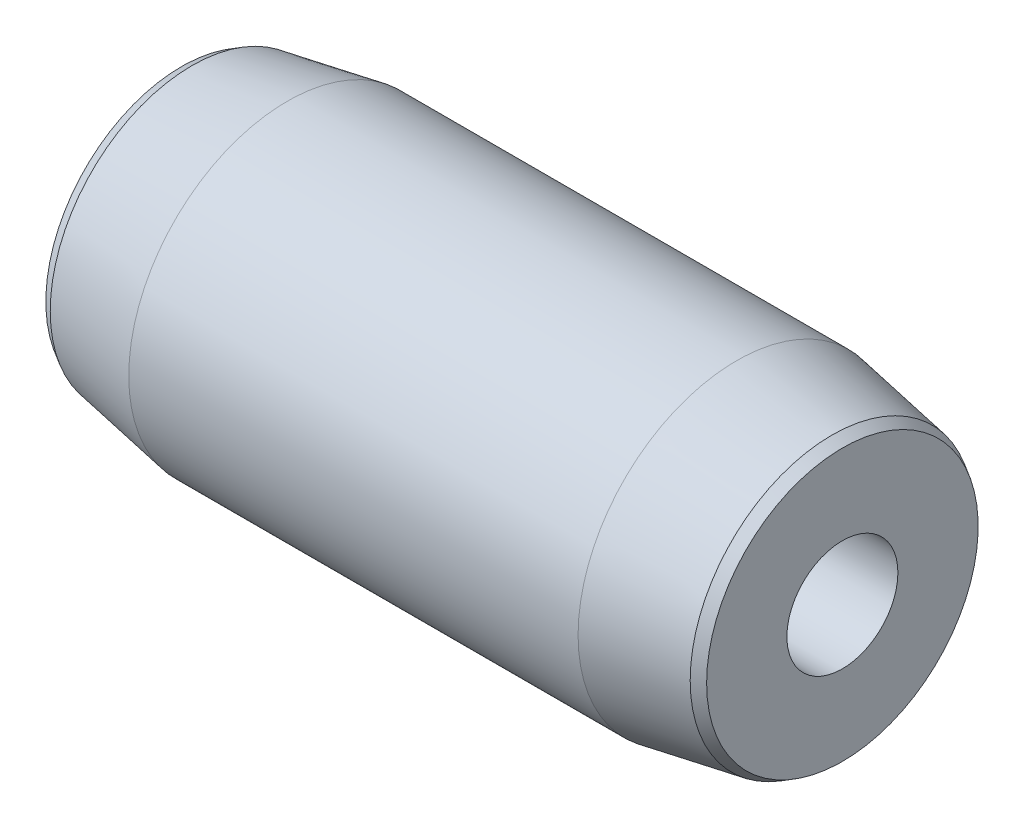
from build123d import *
from OCP.BRepFilletAPI import BRepFilletAPI_MakeChamfer

# Parameters (mm, degrees)
SKETCH_2_R              = 10.5
CUT_EXTRUDE_1_DEPTH     = 133.003787824
HOLE_WIZARD_M24_2_D     = 21
HOLE_WIZARD_M24_2_DEPTH = 63
HOLE_WIZARD_M24_2_TIP   = 6.3090365
CHAMFER_1_SIZE          = 2
CHAMFER_1_SIZE2         = 0.789861687


with BuildPart() as part:
    # 草图1 → 旋转1 (revolve)
    with BuildSketch(Plane.XY, mode=Mode.PRIVATE) as revolve_1_sk:
        Polygon((0, 0), (0, 26.473460386), (20, 30), (105, 30), (125, 26.473460386), (125, 0), align=None)
    revolve(revolve_1_sk.sketch.rotate(Axis((0, 0, 0), (1, 0, 0)), 90), axis=Axis((0, 0, 0), (1, 0, 0)))

    # 草图2 → 切除-拉伸1 (cut, through all)
    with BuildSketch(Plane(origin=(125, 0, 0), x_dir=(0, 0, -1), z_dir=(1, 0, 0))):
        Circle(SKETCH_2_R)
    extrude(amount=-CUT_EXTRUDE_1_DEPTH, mode=Mode.SUBTRACT)

    # M24 螺纹孔2
    with Locations(Plane(origin=(0, 0, 0), x_dir=(0, 0, -1), z_dir=(-1, 0, 0))):
        with Locations((0, 0)):
            Hole(HOLE_WIZARD_M24_2_D / 2, depth=HOLE_WIZARD_M24_2_DEPTH)
            with Locations((0, 0, -(HOLE_WIZARD_M24_2_DEPTH + HOLE_WIZARD_M24_2_TIP / 2))):  # 118° drill point
                Cone(0, HOLE_WIZARD_M24_2_D / 2, HOLE_WIZARD_M24_2_TIP, mode=Mode.SUBTRACT)

    # 倒角1: one chamfer whose edges measure the first distance from different faces: ONE call of the kernel's chamfer builder (chamfer() names one face for all edges)
    chamfer_1_edges_1 = [part.edges().sort_by_distance(p)[0] for p in [
        (0, 0, -26.473460386),
    ]]
    chamfer_1_side_1 = [part.faces().sort_by_distance(p)[0] for p in [
        (10, 0, -28.236730193),
    ]]
    chamfer_1_edges_2 = [part.edges().sort_by_distance(p)[0] for p in [
        (125, 0, -26.473460386),
    ]]
    chamfer_1_side_2 = [part.faces().sort_by_distance(p)[0] for p in [
        (115, 0, -28.236730193),
    ]]
    chamfer_1 = BRepFilletAPI_MakeChamfer(part.part.solid().wrapped)
    for e in chamfer_1_edges_1:
        chamfer_1.Add(CHAMFER_1_SIZE, CHAMFER_1_SIZE2, e.wrapped, chamfer_1_side_1[0].wrapped)  # the first distance lies on this face
    for e in chamfer_1_edges_2:
        chamfer_1.Add(CHAMFER_1_SIZE, CHAMFER_1_SIZE2, e.wrapped, chamfer_1_side_2[0].wrapped)  # the first distance lies on this face
    add(Compound.cast(chamfer_1.Shape()), mode=Mode.REPLACE)


solid = part.part
